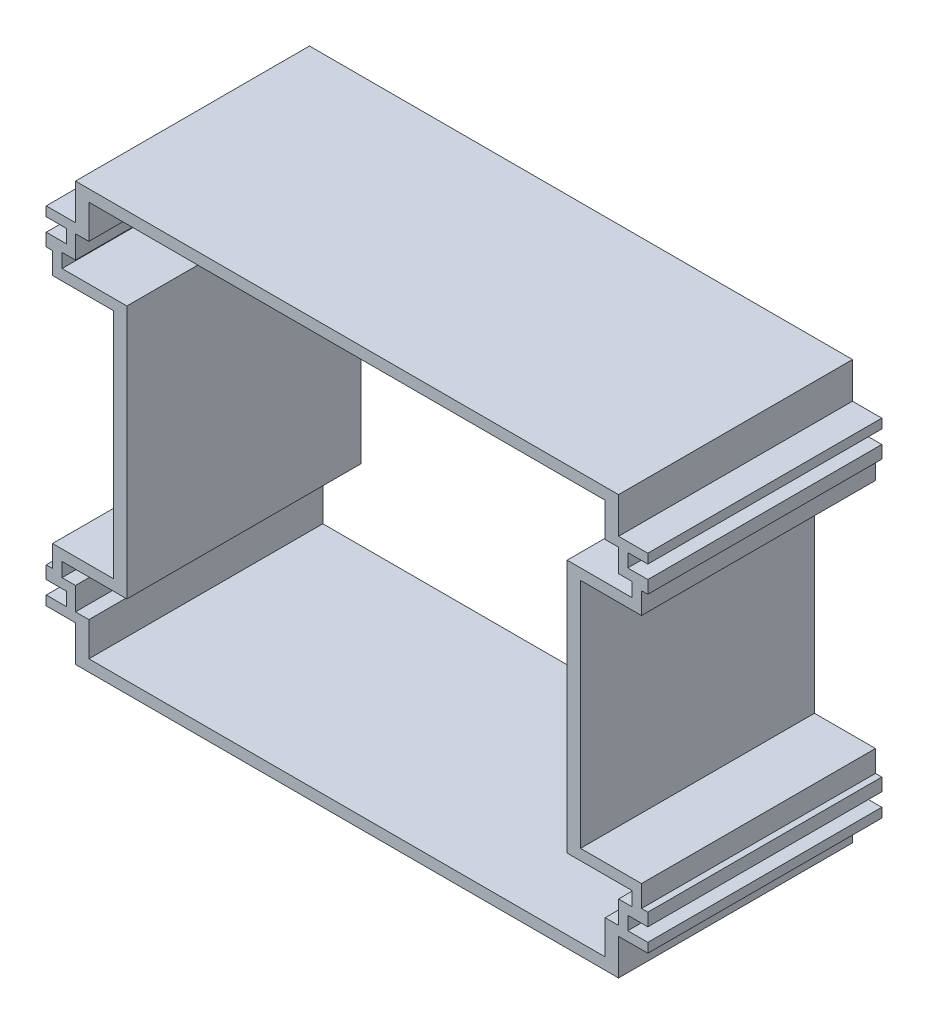
SolidWorks part; units mm, degrees
ref_plane "Front Plane" through (0, 0, 0) normal (0, 0, 1) x (1, 0, 0)
ref_plane "Top Plane" through (0, 0, 0) normal (0, 1, 0) x (1, 0, 0)
ref_plane "Right Plane" through (0, 0, 0) normal (1, 0, 0) x (0, 0, -1)
sketch "Sketch1" plane through (0, 0, 0) normal (0, 0, 1) x (1, 0, 0)
  line L0 (90, 49) -> (84, 49)
  line L1 (84, 49) -> (96, 49) construction
  line L2 (84, 49) -> (84, 45)
  line L3 (84, 45) -> (90, 45)
  line L4 (84, 45) -> (96, 45) construction
  line L5 (90, 45) -> (90, 41.1819)
  line L6 (90, 41.1819) -> (88.1069, 41.1819)
  line L7 (88.1069, 41.1819) -> (88.1069, 34.7197)
  line L8 (88.1069, 34.7197) -> (69.8608, 34.7197)
  line L9 (69.8608, 34.7197) -> (69.8608, -34.7197)
  line L10 (0, 0) -> (0, -7.3888) construction
  line L11 (65.8608, -37.9508) -> (65.8608, 37.9508)
  line L12 (65.8608, 37.9508) -> (85.2615, 37.9508)
  line L13 (85.2615, 37.9508) -> (85.2615, 42.1475)
  line L14 (85.2615, 42.1475) -> (81.2401, 42.1475)
  line L15 (81.2401, 42.1475) -> (81.2401, 49)
  line L16 (81.2401, 51.8274) -> (90, 51.8274)
  line L17 (90, 51.8274) -> (90, 49)
  line L18 (90, -51.8274) -> (90, -49)
  line L19 (81.2401, -51.8274) -> (90, -51.8274)
  line L20 (81.2401, -42.1475) -> (81.2401, -49)
  line L21 (85.2615, -42.1475) -> (81.2401, -42.1475)
  line L22 (85.2615, -37.9508) -> (85.2615, -42.1475)
  line L23 (65.8608, -37.9508) -> (85.2615, -37.9508)
  line L24 (88.1069, -34.7197) -> (69.8608, -34.7197)
  line L25 (88.1069, -41.1819) -> (88.1069, -34.7197)
  line L26 (90, -41.1819) -> (88.1069, -41.1819)
  line L27 (90, -45) -> (90, -41.1819)
  line L28 (84, -45) -> (90, -45)
  line L29 (84, -49) -> (84, -45)
  line L30 (90, -49) -> (84, -49)
  line L31 (-90, -49) -> (-84, -49)
  line L32 (-84, -49) -> (-84, -45)
  line L33 (-84, -45) -> (-90, -45)
  line L34 (-90, -45) -> (-90, -41.1819)
  line L35 (-90, -41.1819) -> (-88.1069, -41.1819)
  line L36 (-88.1069, -41.1819) -> (-88.1069, -34.7197)
  line L37 (-88.1069, -34.7197) -> (-69.8608, -34.7197)
  line L38 (-65.8608, -37.9508) -> (-85.2615, -37.9508)
  line L39 (-85.2615, -37.9508) -> (-85.2615, -42.1475)
  line L40 (-85.2615, -42.1475) -> (-81.2401, -42.1475)
  line L41 (-81.2401, -42.1475) -> (-81.2401, -49)
  line L42 (-81.2401, -51.8274) -> (-90, -51.8274)
  line L43 (-90, -51.8274) -> (-90, -49)
  line L44 (-90, 51.8274) -> (-90, 49)
  line L45 (-81.2401, 51.8274) -> (-90, 51.8274)
  line L46 (-81.2401, 42.1475) -> (-81.2401, 49)
  line L47 (-85.2615, 42.1475) -> (-81.2401, 42.1475)
  line L48 (-85.2615, 37.9508) -> (-85.2615, 42.1475)
  line L49 (-65.8608, 37.9508) -> (-85.2615, 37.9508)
  line L50 (-65.8608, -37.9508) -> (-65.8608, 37.9508)
  line L51 (-69.8608, 34.7197) -> (-69.8608, -34.7197)
  line L52 (-88.1069, 34.7197) -> (-69.8608, 34.7197)
  line L53 (-88.1069, 41.1819) -> (-88.1069, 34.7197)
  line L54 (-90, 41.1819) -> (-88.1069, 41.1819)
  line L55 (-90, 45) -> (-90, 41.1819)
  line L56 (-84, 45) -> (-90, 45)
  line L57 (-84, 49) -> (-84, 45)
  line L58 (-90, 49) -> (-84, 49)
  line L59 (81.2401, 51.8274) -> (81.2401, 62.6262)
  line L60 (81.2401, 62.6262) -> (-81.2401, 62.6262)
  line L61 (-81.2401, 62.6262) -> (-81.2401, 51.8274)
  line L62 (81.2401, 49) -> (77.2401, 49)
  line L63 (77.2401, 49) -> (77.2401, 59.1638)
  line L64 (77.2401, 59.1638) -> (-77.2401, 59.1638)
  line L65 (-77.2401, 59.1638) -> (-77.2401, 49)
  line L66 (-77.2401, 49) -> (-81.2401, 49)
  line L67 (0, 0) -> (-7.913, 0) construction
  line L68 (-77.2401, -59.1638) -> (-77.2401, -49)
  line L69 (77.2401, -59.1638) -> (-77.2401, -59.1638)
  line L70 (77.2401, -49) -> (77.2401, -59.1638)
  line L71 (-81.2401, -62.6262) -> (-81.2401, -51.8274)
  line L72 (81.2401, -62.6262) -> (-81.2401, -62.6262)
  line L73 (81.2401, -51.8274) -> (81.2401, -62.6262)
  line L74 (81.2401, -49) -> (77.2401, -49)
  line L75 (-77.2401, -49) -> (-81.2401, -49)
  dimension "D1" = 4
  dimension "D2" = 4
extrude "Boss-Extrude1" add sketch "Sketch1" against normal up to vertex (104.5623 mm away) contours L64 L65 L66 L46 L47 L48 L49 L50 L38 L39 L40 L41 L75 L68 L69 L70 L74 L20 L21 L22 L23 L11 L12 L13 L14 L15 L62 L63
